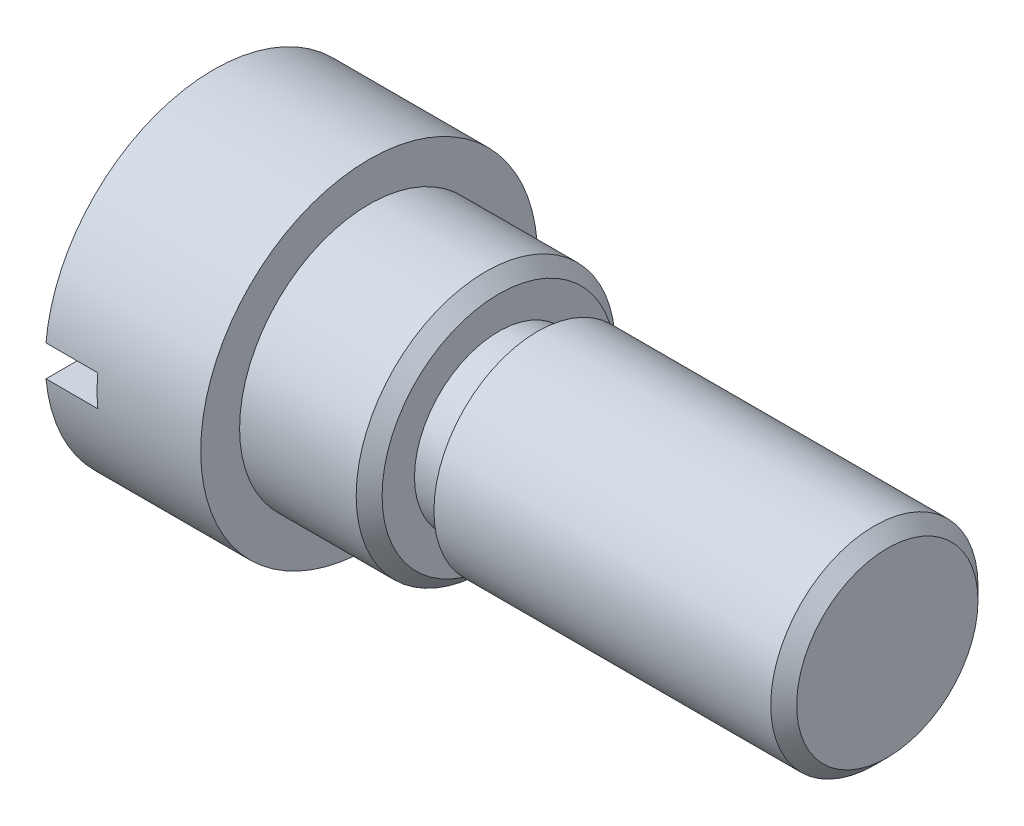
from build123d import *

# Parameters (mm, degrees)
SKETCH_2_R          = 5
EXTRUDE_1_DEPTH     = 5
SKETCH_5_R          = 6.5
EXTRUDE_2_DEPTH     = 6
SKETCH_6_W          = 30
SKETCH_6_H          = 1.2
CUT_EXTRUDE_1_DEPTH = 2
SKETCH_7_R          = 4
EXTRUDE_3_DEPTH     = 15
CHAMFER_3_SIZE      = 0.5
SKETCH_8_W          = 1.5
SKETCH_8_H          = 1.794916968


with BuildPart() as part:
    # 草图2 → 凸台-拉伸1 (new body)
    with BuildSketch(Plane(origin=(0, 0, 0), x_dir=(0, 0, -1), z_dir=(1, 0, 0))):
        Circle(SKETCH_2_R)
    extrude(amount=EXTRUDE_1_DEPTH)

    # 草图5 → 凸台-拉伸2 (add)
    with BuildSketch(Plane.ZY):
        Circle(SKETCH_5_R)
    extrude(amount=EXTRUDE_2_DEPTH)

    # 草图6 → 切除-拉伸1 (cut)
    with BuildSketch(Plane.ZY.offset(6)):
        Rectangle(SKETCH_6_W, SKETCH_6_H)
    extrude(amount=-CUT_EXTRUDE_1_DEPTH, mode=Mode.SUBTRACT)

    # 草图7 → 凸台-拉伸3 (add)
    with BuildSketch(Plane(origin=(5, 0, 0), x_dir=(0, 0, -1), z_dir=(1, 0, 0))):
        Circle(SKETCH_7_R)
    extrude(amount=EXTRUDE_3_DEPTH)

    # 倒角3
    chamfer_3_edges = [part.edges().sort_by_distance(p)[0] for p in [
        (20, 0, 4),
        (5, 0, 5),
    ]]
    chamfer(chamfer_3_edges, length=CHAMFER_3_SIZE)

    # 草图8 → 切除-旋转1 (revolve, cut)
    with BuildSketch(Plane(origin=(0, 0, 0), x_dir=(1, 0, 0), z_dir=(0, 1, 0)), mode=Mode.PRIVATE) as cut_revolve_1_sk:
        with Locations((5.75, 4.147458484)):
            Rectangle(SKETCH_8_W, SKETCH_8_H)
    revolve(cut_revolve_1_sk.sketch.rotate(Axis((0, 0, 0), (1, 0, 0)), 180), axis=Axis((0, 0, 0), (1, 0, 0)), mode=Mode.SUBTRACT)


solid = part.part
